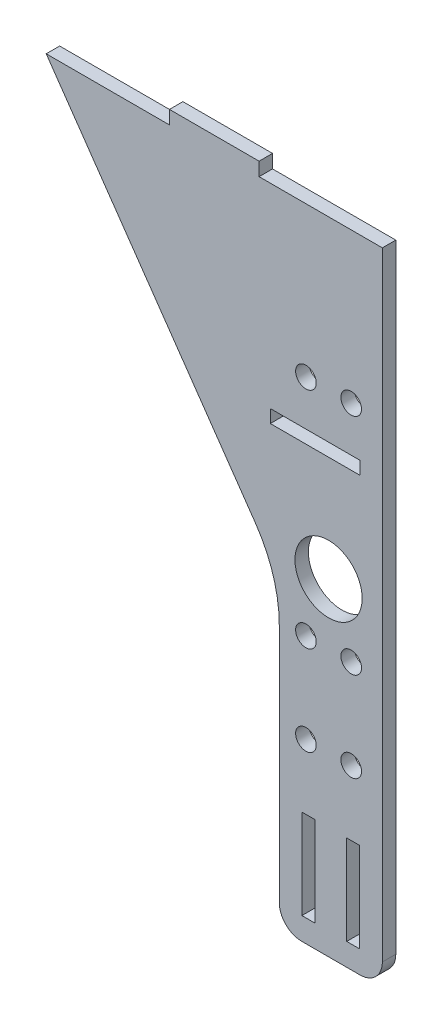
from build123d import *

# Parameters (mm, degrees)
SKETCH1_W           = 2.9
SKETCH1_H           = 20
BOSS_EXTRUDE1_DEPTH = 3
FILLET1_R           = 5
FILLET2_R           = 30
CUT_EXTRUDE1_REACH  = 166.165
SKETCH3_R           = 7.5
SKETCH3_R_2         = 2.3
SKETCH5_W           = 20
SKETCH5_H           = 2.9
CUT_EXTRUDE2_DEPTH  = 3
SKETCH6_R           = 2.3
CUT_EXTRUDE3_DEPTH  = 3


with BuildPart() as part:
    # Sketch1 → Boss-Extrude1 (new body)
    with BuildSketch(Plane.XY):
        Polygon((0, 0), (-23, 0), (-23, 68), (-75, 143), (-47.5, 143), (-47.5, 146), (-27.5, 146), (-27.5, 143), (0, 143), align=None)
        with Locations((-16.5, 15)):
            Rectangle(SKETCH1_W, SKETCH1_H, mode=Mode.SUBTRACT)
        with Locations((-6.5, 15)):
            Rectangle(SKETCH1_W, SKETCH1_H, mode=Mode.SUBTRACT)
    extrude(amount=BOSS_EXTRUDE1_DEPTH)

    # Fillet1
    fillet1_edges = [part.edges().sort_by_distance(p)[0] for p in [
        (0, 0, 1.5),
        (-23, 0, 1.5),
    ]]
    fillet(fillet1_edges, radius=FILLET1_R)

    # Fillet2
    fillet2_edges = [part.edges().sort_by_distance(p)[0] for p in [
        (-23, 68, 1.5),
    ]]
    fillet(fillet2_edges, radius=FILLET2_R)

    # Sketch3 → Cut-Extrude1 (cut, up to next)
    with BuildSketch(Plane(origin=(0, 0, 0), x_dir=(-1, 0, 0), z_dir=(0, 0, -1)), mode=Mode.PRIVATE) as cut_extrude1_sk1:
        with Locations((12, 73)):
            Circle(SKETCH3_R)
    cut_extrude1_tool1 = extrude(cut_extrude1_sk1.sketch, amount=-CUT_EXTRUDE1_REACH, mode=Mode.PRIVATE) & part.part
    # Sketch3 → Cut-Extrude1 (cut, up to next)
    with BuildSketch(Plane(origin=(0, 0, 0), x_dir=(-1, 0, 0), z_dir=(0, 0, -1)), mode=Mode.PRIVATE) as cut_extrude1_sk2:
        with Locations((17.05, 59.5)):
            Circle(SKETCH3_R_2)
    cut_extrude1_tool2 = extrude(cut_extrude1_sk2.sketch, amount=-CUT_EXTRUDE1_REACH, mode=Mode.PRIVATE) & part.part
    # Sketch3 → Cut-Extrude1 (cut, up to next)
    with BuildSketch(Plane(origin=(0, 0, 0), x_dir=(-1, 0, 0), z_dir=(0, 0, -1)), mode=Mode.PRIVATE) as cut_extrude1_sk3:
        with Locations((6.95, 59.5)):
            Circle(SKETCH3_R_2)
    cut_extrude1_tool3 = extrude(cut_extrude1_sk3.sketch, amount=-CUT_EXTRUDE1_REACH, mode=Mode.PRIVATE) & part.part
    # Sketch3 → Cut-Extrude1 (cut, up to next)
    with BuildSketch(Plane(origin=(0, 0, 0), x_dir=(-1, 0, 0), z_dir=(0, 0, -1)), mode=Mode.PRIVATE) as cut_extrude1_sk4:
        with Locations((17.05, 109.5)):
            Circle(SKETCH3_R_2)
    cut_extrude1_tool4 = extrude(cut_extrude1_sk4.sketch, amount=-CUT_EXTRUDE1_REACH, mode=Mode.PRIVATE) & part.part
    # Sketch3 → Cut-Extrude1 (cut, up to next)
    with BuildSketch(Plane(origin=(0, 0, 0), x_dir=(-1, 0, 0), z_dir=(0, 0, -1)), mode=Mode.PRIVATE) as cut_extrude1_sk5:
        with Locations((6.95, 109.5)):
            Circle(SKETCH3_R_2)
    cut_extrude1_tool5 = extrude(cut_extrude1_sk5.sketch, amount=-CUT_EXTRUDE1_REACH, mode=Mode.PRIVATE) & part.part
    add(cut_extrude1_tool1.solids().sort_by_distance((-12, 73, 0))[0], mode=Mode.SUBTRACT)
    add(cut_extrude1_tool2.solids().sort_by_distance((-17.05, 59.5, 0))[0], mode=Mode.SUBTRACT)
    add(cut_extrude1_tool3.solids().sort_by_distance((-6.95, 59.5, 0))[0], mode=Mode.SUBTRACT)
    add(cut_extrude1_tool4.solids().sort_by_distance((-17.05, 109.5, 0))[0], mode=Mode.SUBTRACT)
    add(cut_extrude1_tool5.solids().sort_by_distance((-6.95, 109.5, 0))[0], mode=Mode.SUBTRACT)

    # Sketch5 → Cut-Extrude2 (cut)
    with BuildSketch(Plane(origin=(0, 0, 0), x_dir=(-1, 0, 0), z_dir=(0, 0, -1))):
        with Locations((15, 98)):
            Rectangle(SKETCH5_W, SKETCH5_H)
    extrude(amount=-CUT_EXTRUDE2_DEPTH, mode=Mode.SUBTRACT)

    # Sketch6 → Cut-Extrude3 (cut)
    with BuildSketch(Plane.XY.offset(3)):
        with Locations((-17.05, 39.5)):
            Circle(SKETCH6_R)
        with Locations((-6.95, 39.5)):
            Circle(SKETCH6_R)
    extrude(amount=-CUT_EXTRUDE3_DEPTH, mode=Mode.SUBTRACT)


solid = part.part
